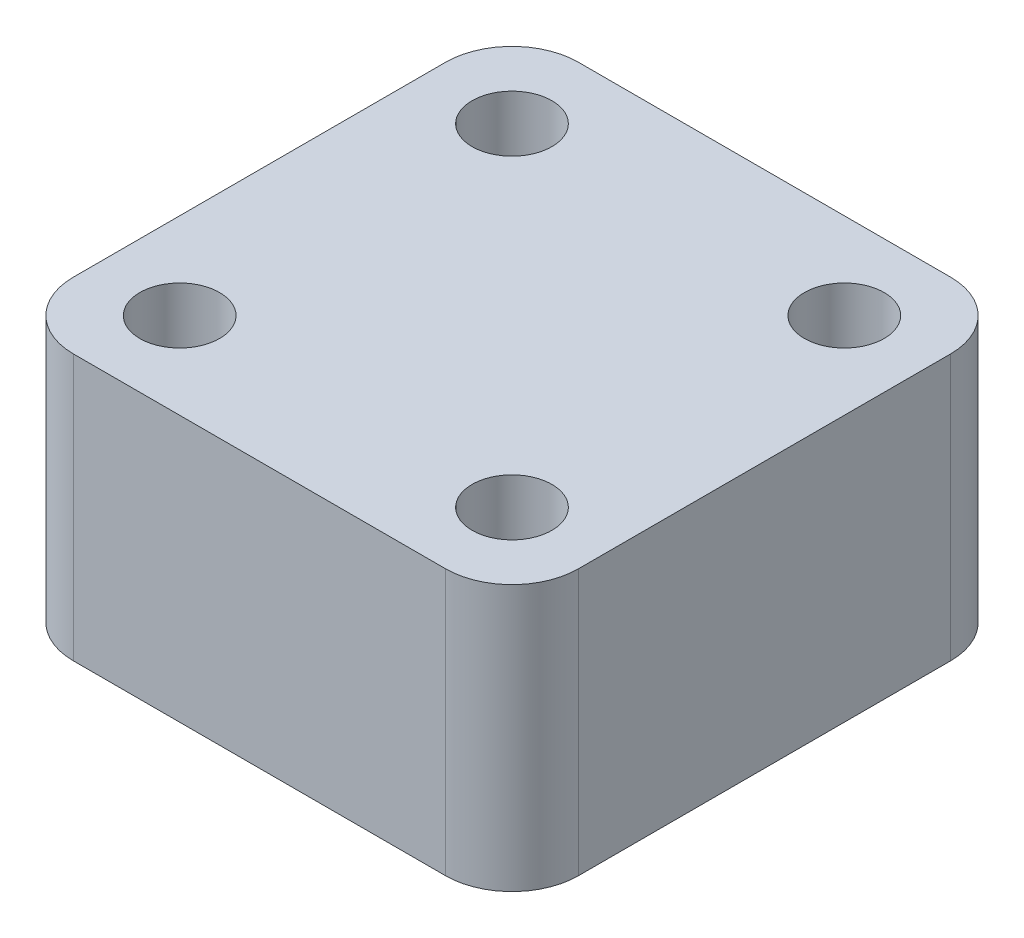
SolidWorks part; units mm, degrees
material "聚氨脂"
ref_plane "Front Plane" through (0, 0, 0) normal (0, 0, 1) x (1, 0, 0)
ref_plane "Top Plane" through (0, 0, 0) normal (0, 1, 0) x (1, 0, 0)
ref_plane "Right Plane" through (0, 0, 0) normal (1, 0, 0) x (0, 0, -1)
sketch "Sketch1" plane through (0, 0, 0) normal (0, 1, 0) x (1, 0, 0)
  line L1 (-14, 19) -> (14, 19)
  line L2 (-19, 14) -> (-19, -14)
  line L3 (-14, -19) -> (14, -19)
  line L4 (19, 14) -> (19, -14)
  line L5 (-19, 19) -> (19, -19) construction
  line L6 (-19, -19) -> (19, 19) construction
  arc A0 (14, 19) -> (19, 14) centre (14, 14) cw
  arc A1 (-14, 19) -> (-19, 14) centre (-14, 14) ccw
  arc A2 (-19, -14) -> (-14, -19) centre (-14, -14) ccw
  arc A3 (14, -19) -> (19, -14) centre (14, -14) ccw
  point P0 (0, 0)
  dimension "D3" = 5
  dimension "D1" = 38
  dimension "D2" = 38
extrude "Boss-Extrude1" add sketch "Sketch1" along normal blind 20
hole_wizard "Hole size (%based on) socket head cap screw type 1" positions "Sketch2" profile "Sketch3" counterbore size "M3" standard "GB" end condition through all
sketch "Sketch2" plane through (0, 20, 0) normal (0, 1, 0) x (1, 0, 0)
  line L0 (-12.5, 12.5) -> (12.5, 12.5)
  line L1 (12.5, 12.5) -> (12.5, -12.5)
  line L2 (12.5, -12.5) -> (-12.5, -12.5)
  line L3 (-12.5, -12.5) -> (-12.5, 12.5)
  line L5 (0, 0) -> (-12.5, 0)
  line L7 (0, 0) -> (0, 12.5)
  point P21 (-12.5, 12.5)
  point P23 (12.5, 12.5)
  point P25 (12.5, -12.5)
  point P27 (-12.5, -12.5)
  dimension "D1" = 25
  dimension "D2" = 25
sketch "Sketch3" plane through (-12.5, 20, -12.5) normal (1, 0, 0) x (0, 0, 1)
  line L0 (0, 0) -> (0, 20)
  line L1 (0, 20) -> (1.7, 20)
  line L3 (1.7, 20) -> (1.7, 10)
  line L4 (1.7, 10) -> (3, 10)
  line L5 (3, 10) -> (3, 0)
  line L7 (3, 0) -> (0, 0)
  line L11 (0, -6.35) -> (0, 107.95) construction
  dimension "通孔孔直径" = 3.4
  dimension "通孔孔深度" = 20
  dimension "柱形沉头孔直径" = 6
  dimension "柱形沉头孔深度" = 10
